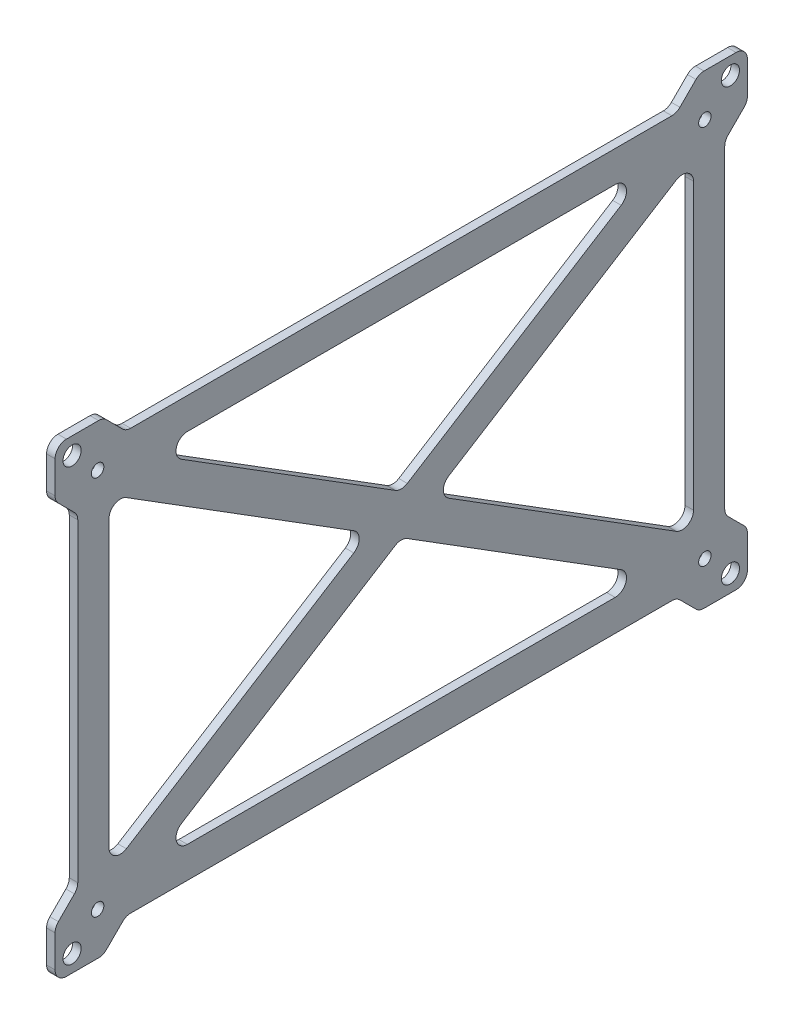
SolidWorks part; units mm, degrees
material "Thornel Mat VMA"
ref_plane "前视基准面" through (0, 0, 0) normal (0, 0, 1) x (1, 0, 0)
ref_plane "上视基准面" through (0, 0, 0) normal (0, 1, 0) x (1, 0, 0)
ref_plane "右视基准面" through (0, 0, 0) normal (1, 0, 0) x (0, 0, -1)
other "Configuration Table"
sketch "草图1" plane through (0, 0, 0) normal (1, 0, 0) x (0, 0, -1)
  line L1 (0, 0) -> (116, 0) construction
  line L2 (0, 0) -> (0, 76) construction
  line L3 (0, 76) -> (116, 76) construction
  line L4 (116, 0) -> (116, 76) construction
  line L5 (4.5, 71.5) -> (111.5, 71.5) construction
  line L6 (4.5, 71.5) -> (4.5, 4.5) construction
  line L7 (4.5, 4.5) -> (111.5, 4.5) construction
  line L8 (111.5, 71.5) -> (111.5, 4.5) construction
  line L9 (-3, 79) -> (119, 79)
  line L10 (-3, 79) -> (-3, -3)
  line L11 (-3, -3) -> (119, -3)
  line L12 (119, 79) -> (119, -3)
  circle A0 centre (0, 76) radius 1.6
  circle A1 centre (0, 0) radius 1.6
  circle A2 centre (116, 76) radius 1.6
  circle A3 centre (116, 0) radius 1.6
  circle A4 centre (4.5, 71.5) radius 1.1
  circle A5 centre (4.5, 4.5) radius 1.1
  circle A6 centre (111.5, 71.5) radius 1.1
  circle A7 centre (111.5, 4.5) radius 1.1
  circle A8 centre (0, 76) radius 2.5 construction
  circle A9 centre (4.5, 71.5) radius 3.1 construction
  dimension "D3" = 3.2
  dimension "D4" = 3.2
  dimension "D5" = 3.2
  dimension "D6" = 3.2
  dimension "D7" = 2.2
  dimension "D8" = 2.2
  dimension "D9" = 2.2
  dimension "D10" = 2.2
  dimension "D13" = 5
  dimension "D16" = 6.2
  dimension "D1" = 76
  dimension "D2" = 116
  dimension "D11" = 107
  dimension "D12" = 67
  dimension "D14" = 4.5
  dimension "D15" = 4.5
  dimension "D17" = 3
  dimension "D18" = 3
  dimension "D19" = 3
  dimension "D20" = 3
extrude "凸台-拉伸1" add sketch "草图1" along normal blind 1.5
sketch "草图2" plane through (1.5, 0, 0) normal (1, 0, 0) x (0, 0, -1)
  line L0 (4.5, 71.5) -> (111.5, 4.5) construction
  line L1 (6.0921, 74.0427) -> (113.0921, 7.0427)
  line L2 (2.9079, 68.9573) -> (109.9079, 1.9573)
  line L3 (4.5, 71.5) -> (4.5, 4.5) construction
  line L4 (6.5, 71.5) -> (6.5, 4.5)
  line L5 (2.5, 71.5) -> (2.5, 4.5)
  line L6 (4.5, 4.5) -> (111.5, 71.5) construction
  line L7 (2.9079, 7.0427) -> (109.9079, 74.0427)
  line L8 (6.0921, 1.9573) -> (113.0921, 68.9573)
  line L9 (111.5, 71.5) -> (4.5, 71.5) construction
  line L10 (111.5, 69.5) -> (4.5, 69.5)
  line L11 (111.5, 73.5) -> (4.5, 73.5)
  line L12 (111.5, 71.5) -> (111.5, 4.5) construction
  line L13 (113.5, 71.5) -> (113.5, 4.5)
  line L14 (109.5, 71.5) -> (109.5, 4.5)
  line L15 (111.5, 4.5) -> (4.5, 4.5) construction
  line L16 (111.5, 2.5) -> (4.5, 2.5)
  line L17 (111.5, 6.5) -> (4.5, 6.5)
  arc A0 (6.0921, 74.0427) -> (2.9079, 68.9573) centre (4.5, 71.5) ccw
  arc A1 (109.9079, 1.9573) -> (113.0921, 7.0427) centre (111.5, 4.5) ccw
  arc A2 (6.5, 71.5) -> (2.5, 71.5) centre (4.5, 71.5) ccw
  arc A3 (2.5, 4.5) -> (6.5, 4.5) centre (4.5, 4.5) ccw
  arc A4 (2.9079, 7.0427) -> (6.0921, 1.9573) centre (4.5, 4.5) ccw
  arc A5 (113.0921, 68.9573) -> (109.9079, 74.0427) centre (111.5, 71.5) ccw
  arc A6 (111.5, 69.5) -> (111.5, 73.5) centre (111.5, 71.5) ccw
  arc A7 (4.5, 73.5) -> (4.5, 69.5) centre (4.5, 71.5) ccw
  arc A8 (113.5, 71.5) -> (109.5, 71.5) centre (111.5, 71.5) ccw
  arc A9 (109.5, 4.5) -> (113.5, 4.5) centre (111.5, 4.5) ccw
  arc A10 (111.5, 2.5) -> (111.5, 6.5) centre (111.5, 4.5) ccw
  arc A11 (4.5, 6.5) -> (4.5, 2.5) centre (4.5, 4.5) ccw
  point P4 (58, 38)
  point P12 (4.5, 38)
  point P20 (58, 38)
  point P27 (58, 71.5)
  point P34 (111.5, 38)
  point P41 (58, 4.5)
  dimension "D1" = 3
  dimension "D2" = 2
  dimension "D3" = 3
  dimension "D4" = 2
  dimension "D5" = 2
  dimension "D6" = 2
extrude "切除-拉伸1" cut sketch "草图2" against normal through all contours L7 L10 L1 | L4 L7 L2 | L17 L2 L8 | L14 L8 L1
sketch "草图3" plane through (1.5, 0, 0) normal (1, 0, 0) x (0, 0, -1)
  line L0 (0, 76) -> (4.5, 71.5) construction
  line L1 (5.4853, 79) -> (9.4853, 75)
  line L2 (119, 79) -> (-3, 79) construction
  line L3 (9.4853, 75) -> (106.5147, 75)
  line L4 (106.5147, 75) -> (110.5147, 79)
  line L5 (110.5147, 79) -> (5.4853, 79)
  line L6 (116, 76) -> (111.5, 71.5) construction
  line L7 (102.6532, 69.5) -> (13.3468, 69.5) construction
  line L8 (-3, 38) -> (52.3472, 38) construction
  line L9 (-3, 79) -> (-3, -3) construction
  line L10 (106.5147, 1) -> (110.5147, -3)
  line L11 (110.5147, -3) -> (5.4853, -3)
  line L12 (9.4853, 1) -> (106.5147, 1)
  line L13 (5.4853, -3) -> (9.4853, 1)
  line L14 (-3, 70.5147) -> (1, 66.5147)
  line L15 (1, 66.5147) -> (1, 9.4853)
  line L16 (1, 9.4853) -> (-3, 5.4853)
  line L17 (-3, 5.4853) -> (-3, 70.5147)
  line L18 (4.5, 4.5) -> (0, 0) construction
  line L19 (6.5, 66.7081) -> (6.5, 9.2919) construction
  line L20 (58, 41.5396) -> (58, 69.5) construction
  line L21 (115, 9.4853) -> (119, 5.4853)
  line L22 (119, 5.4853) -> (119, 70.5147)
  line L23 (115, 66.5147) -> (115, 9.4853)
  line L24 (119, 70.5147) -> (115, 66.5147)
  dimension "D1" = 6
  dimension "D2" = 5.5
  dimension "D3" = 6
  dimension "D4" = 5.5
  dimension "D5" = 6
  dimension "D6" = 6
extrude "切除-拉伸2" cut sketch "草图3" against normal through all
fillet "圆角1" radius 2 32 edges at (0.75, 6.5, -13.3468) (0.75, 34.4604, -58) (0.75, 6.5, -102.6532) (0.75, 38, -52.3472) (0.75, 9.2919, -6.5) (0.75, 75, -9.4853) (0.75, 79, -5.4853) (0.75, 79, 3) (0.75, 70.5147, 3) (0.75, 66.5147, -1) (0.75, 9.4853, -1) (0.75, 5.4853, 3) (0.75, -3, 3) (0.75, -3, -5.4853) (0.75, 1, -9.4853) (0.75, 1, -106.5147) (0.75, -3, -110.5147) (0.75, -3, -119) (0.75, 5.4853, -119) (0.75, 9.4853, -115) (0.75, 66.5147, -115) (0.75, 70.5147, -119) (0.75, 79, -119) (0.75, 79, -110.5147) (0.75, 75, -106.5147) (0.75, 69.5, -13.3468) (0.75, 69.5, -102.6532) (0.75, 41.5396, -58) (0.75, 9.2919, -109.5) (0.75, 38, -63.6528) (0.75, 66.7081, -109.5) (0.75, 66.7081, -6.5)
